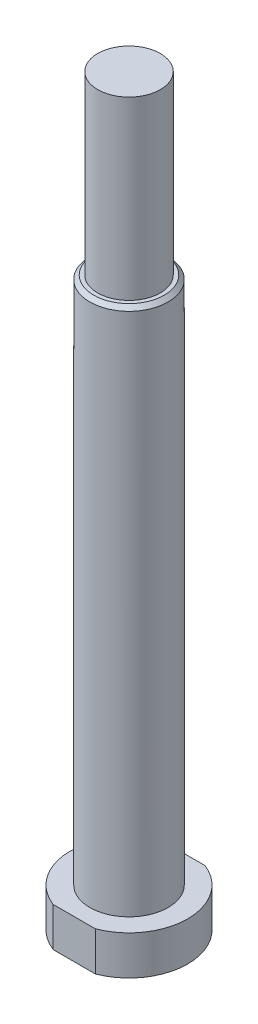
SolidWorks part; units mm, degrees
ref_plane "前视基准面" through (0, 0, 0) normal (0, 0, 1) x (1, 0, 0)
ref_plane "上视基准面" through (0, 0, 0) normal (0, 1, 0) x (1, 0, 0)
ref_plane "右视基准面" through (0, 0, 0) normal (1, 0, 0) x (0, 0, -1)
sketch "草图1" plane through (0, 0, 0) normal (0, 0, 1) x (1, 0, 0)
  line L0 (0, 95) -> (0, -95)
  line L1 (0, -95) -> (15, -95)
  line L2 (15, -95) -> (15, -85)
  line L3 (15, -85) -> (10, -85)
  line L4 (10, -85) -> (10, 50)
  line L5 (10, 50) -> (8, 50)
  line L6 (8, 50) -> (8, 95)
  line L7 (8, 95) -> (0, 95)
  point P4 (0, 0)
  dimension "D1" = 190
  dimension "D2" = 15
  dimension "D3" = 10
  dimension "D4" = 8
  dimension "D5" = 10
  dimension "D6" = 135
revolve "旋转1" add sketch "草图1" angle 360 about L0
cosmetic thread "装饰螺纹线1" parameters "D2"=15
chamfer "倒角1" distance 1 angle 45 1 edges at (-10, 50, 0)
sketch "草图2" plane through (0, -85, 0) normal (0, 1, 0) x (1, 0, 0)
  line L0 (16.9193, -14) -> (-19.9666, -14)
  line L1 (20.4447, 14) -> (-19.9666, 14)
  line L2 (-19.9666, 14) -> (-19.9666, 18.7766)
  line L3 (-19.9666, 18.7766) -> (20.4447, 18.7766)
  line L4 (20.4447, 18.7766) -> (20.4447, 14)
  line L5 (16.9193, -14) -> (16.9193, -18.9263)
  line L6 (16.9193, -18.9263) -> (-19.9666, -18.9263)
  line L7 (-19.9666, -18.9263) -> (-19.9666, -14)
  dimension "D1" = 14
  dimension "D2" = 14
extrude "切除-拉伸1" cut sketch "草图2" against normal blind 30
